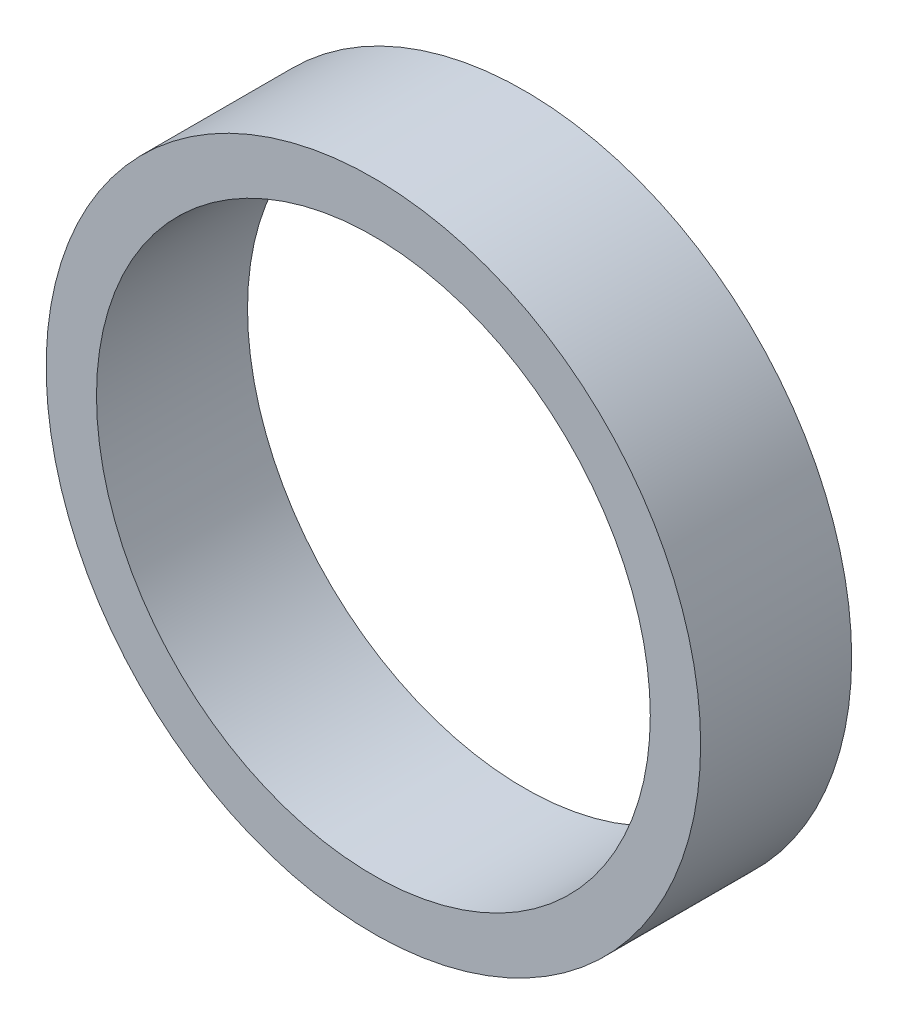
SolidWorks part; units mm, degrees
ref_plane "Front Plane" through (0, 0, 0) normal (0, 0, 1) x (1, 0, 0)
ref_plane "Top Plane" through (0, 0, 0) normal (0, 1, 0) x (1, 0, 0)
ref_plane "Right Plane" through (0, 0, 0) normal (1, 0, 0) x (0, 0, -1)
sketch "Sketch1" plane through (0, 0, 0) normal (0, 0, 1) x (1, 0, 0)
  circle A0 centre (0, 0) radius 11
  circle A1 centre (0, 0) radius 13
  dimension "D1" = 26
  dimension "D2" = 22
extrude "Boss-Extrude1" add sketch "Sketch1" along normal blind 6
